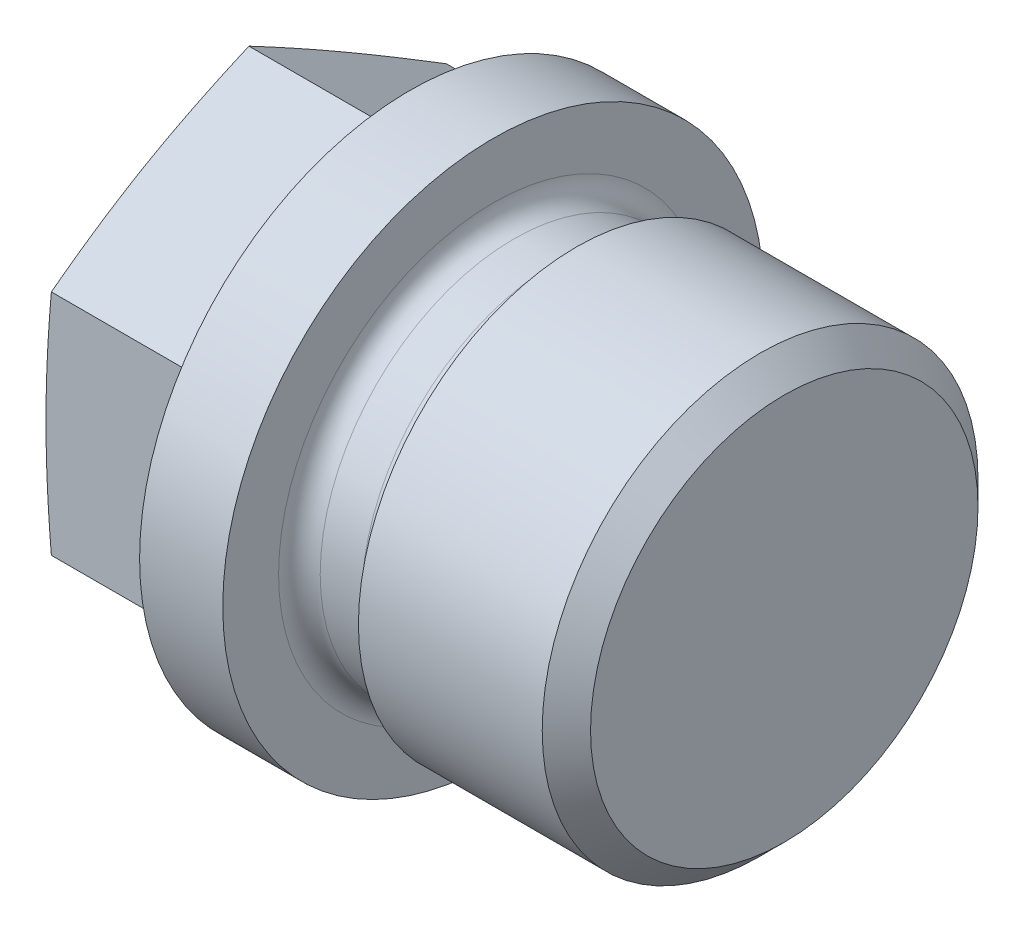
from build123d import *

# Parameters (mm, degrees)
EXTRUDE1_DEPTH     = 8
SKETCH3_OUTSIDE_W  = 150.432
SKETCH3_OUTSIDE_H  = 150.432
SKETCH3_OUTSIDE_R  = 9.5
CUT_EXTRUDE1_DEPTH = 10
CUT_EXTRUDE1_DRAFT = -80
FILLET1_R          = 1


with BuildPart() as part:
    # Sketch1 → Revolve1 (revolve)
    with BuildSketch(Plane.XY, mode=Mode.PRIVATE) as revolve1_sk:
        Polygon((16, 10.4775), (16, 9.3155), (12, 9.3155), (12, 13), (8, 13), (8, 1.5), (0, 1.5), (0, 0), (26, 0), (26, 9.3155), (24.838, 10.4775), align=None)
    revolve(revolve1_sk.sketch.rotate(Axis((0, 0, 0), (1, 0, 0)), 90), axis=Axis((0, 0, 0), (1, 0, 0)))

    # Sketch2 → Extrude1 (add)
    with BuildSketch(Plane.ZY):
        Polygon((0, 10.969655115), (-9.5, 5.484827557), (-9.5, -5.484827557), (0, -10.969655115), (9.5, -5.484827557), (9.5, 5.484827557), align=None)
    extrude(amount=-EXTRUDE1_DEPTH)


with BuildPart() as cut_extrude1_tool:
    # Sketch3 outside → Cut-Extrude1 (with draft: the straight prism first)
    with BuildSketch(Plane.ZY):
        Rectangle(SKETCH3_OUTSIDE_W, SKETCH3_OUTSIDE_H)
        Circle(SKETCH3_OUTSIDE_R, mode=Mode.SUBTRACT)
    extrude(amount=-CUT_EXTRUDE1_DEPTH)
    # Cut-Extrude1: the draft: its side faces are tilted about the plane it starts from
    cut_extrude1_sides = [cut_extrude1_tool.faces().sort_by_distance(p)[0] for p in [
        (5, -75.216, 0),
        (5, 0, 75.216),
        (5, 75.216, 0),
        (5, 0, -75.216),
        (5, 0, -9.5),
    ]]
    draft(cut_extrude1_sides, Plane.ZY, CUT_EXTRUDE1_DRAFT)


with BuildPart() as part_1:
    add(part.part)

    # Cut-Extrude1: cut by cut_extrude1_tool
    add(cut_extrude1_tool.part, mode=Mode.SUBTRACT)

    # Fillet1
    fillet1_edges = [part_1.edges().sort_by_distance(p)[0] for p in [
        (16, 0, -9.3155),
        (12, 0, -9.3155),
    ]]
    fillet(fillet1_edges, radius=FILLET1_R)


solid = part_1.part
